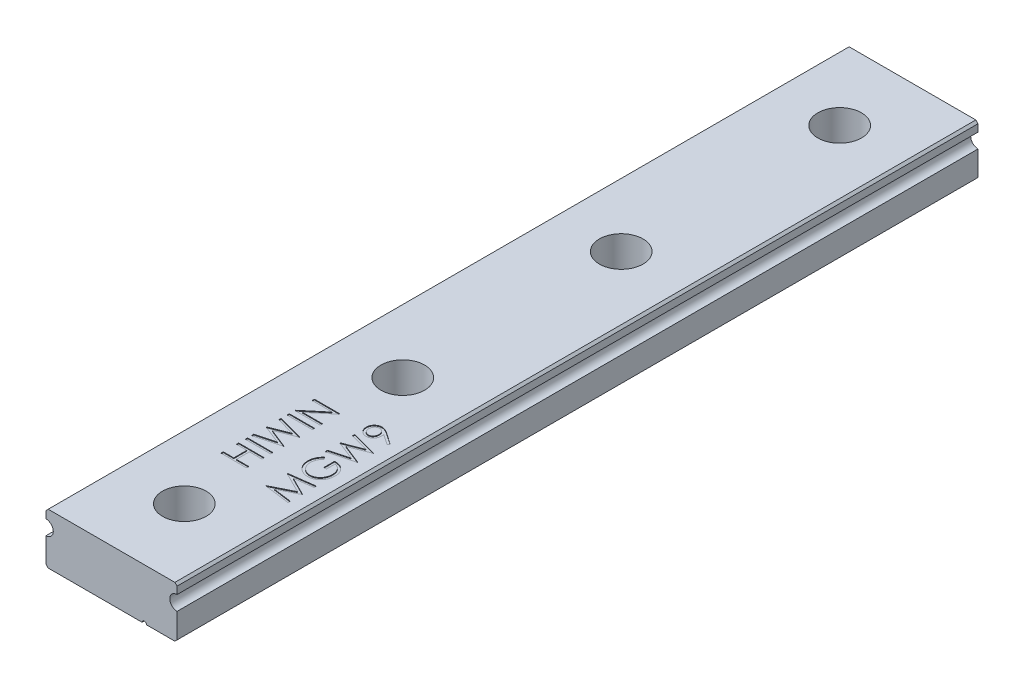
from build123d import *

# Parameters (mm, degrees)
BOSS_EXTRUDE1_DEPTH                                 = 110
CBORE_FOR_M3_HEX_SOCKET_HEAD_CAP_SCREW1_D           = 3.5
CBORE_FOR_M3_HEX_SOCKET_HEAD_CAP_SCREW1_CBORE_D     = 6
CBORE_FOR_M3_HEX_SOCKET_HEAD_CAP_SCREW1_CBORE_DEPTH = 4.5
LPATTERN1_COUNT                                     = 4
LPATTERN1_PITCH                                     = 30
SKETCH4_W                                           = 3.5
SKETCH4_H                                           = 0.314102564
CUT_EXTRUDE1_DEPTH                                  = 0.1


with BuildPart() as part:
    # Sketch1 → Boss-Extrude1 (new body)
    with BuildSketch(Plane.XY):
        with BuildLine():
            Line((9, 5.7), (9, 6.7))
            Line((9, 6.7), (8.7, 7))
            Line((8.7, 7), (-8.7, 7))
            Line((-8.7, 7), (-9, 6.7))
            Line((-9, 6.7), (-9, 5.7))
            ThreePointArc((-9, 5.7), (-8, 4.7), (-9, 3.7))
            Line((-9, 3.7), (-9, 0.3))
            Line((-9, 0.3), (-8.7, 0))
            Line((-8.7, 0), (4.2, 0))
            ThreePointArc((4.2, 0), (4.5, 0.3), (4.8, 0))
            Line((4.8, 0), (8.7, 0))
            Line((8.7, 0), (9, 0.3))
            Line((9, 0.3), (9, 3.7))
            ThreePointArc((9, 3.7), (8, 4.7), (9, 5.7))
        make_face()
    extrude(amount=-BOSS_EXTRUDE1_DEPTH)

    # CBORE for M3 Hex Socket Head Cap Screw1 (through all)
    with Locations(Plane(origin=(-0.084506888, 7, -67.993710711), x_dir=(-1, 0, 0), z_dir=(0, 1, 0))):
        with Locations((-0.084506888, 57.993710711)):
            cbore_for_m3_hex_socket_head_cap_screw1 = CounterBoreHole(CBORE_FOR_M3_HEX_SOCKET_HEAD_CAP_SCREW1_D / 2, CBORE_FOR_M3_HEX_SOCKET_HEAD_CAP_SCREW1_CBORE_D / 2, CBORE_FOR_M3_HEX_SOCKET_HEAD_CAP_SCREW1_CBORE_DEPTH)

    # LPattern1: CBORE for M3 Hex Socket Head Cap Screw1 ×4
    with Locations(*[(0, 0, -i * LPATTERN1_PITCH) for i in range(1, LPATTERN1_COUNT)]):
        add(cbore_for_m3_hex_socket_head_cap_screw1, mode=Mode.SUBTRACT)

    # Sketch4 → Cut-Extrude1 (cut)
    # profile 1 of 9: a face of its own
    with BuildSketch(Plane(origin=(0, 7, 0), x_dir=(1, 0, 0), z_dir=(0, 1, 0))):
        Polygon((-3.5, 18.538461538), (-3.5, 18.852564103), (-2.064102564, 18.852564103), (-2.064102564, 20.647435897), (-3.5, 20.647435897), (-3.5, 20.961538462), (0, 20.961538462), (0, 20.647435897), (-1.705128205, 20.647435897), (-1.705128205, 18.852564103), (0, 18.852564103), (0, 18.538461538), align=None)
    # profile 2 of 9: a face of its own
    with BuildSketch(Plane(origin=(0, 7, 0), x_dir=(1, 0, 0), z_dir=(0, 1, 0))):
        with Locations((-1.75, 22.016025641)):
            Rectangle(SKETCH4_W, SKETCH4_H)
    # profile 3 of 9: a face of its own
    with BuildSketch(Plane(origin=(0, 7, 0), x_dir=(1, 0, 0), z_dir=(0, 1, 0))):
        Polygon((-3.5, 22.711538462), (-3.5, 23.036157853), (-0.933193109, 23.721153846), (-3.5, 24.739883814), (-3.5, 24.785456731), (-0.950721154, 25.78525641), (-3.5, 26.473758013), (-3.5, 26.794871795), (0, 25.851161859), (0, 25.806290064), (-2.676883013, 24.753205128), (0, 23.6875), (0, 23.642628205), align=None)
    # profile 4 of 9: a face of its own
    with BuildSketch(Plane(origin=(0, 7, 0), x_dir=(1, 0, 0), z_dir=(0, 1, 0))):
        with Locations((-1.75, 27.759615385)):
            Rectangle(SKETCH4_W, SKETCH4_H)
    # profile 5 of 9: a face of its own
    with BuildSketch(Plane(origin=(0, 7, 0), x_dir=(1, 0, 0), z_dir=(0, 1, 0))):
        Polygon((0, 28.679487179), (-3.5, 28.679487179), (-3.5, 28.745392628), (-0.745292468, 31.057692308), (-3.5, 31.057692308), (-3.5, 31.371794872), (0, 31.371794872), (0, 31.300280449), (-2.748397436, 28.993589744), (0, 28.993589744), align=None)
    # profile 6 of 9: a face of its own
    with BuildSketch(Plane(origin=(0, 7, 0), x_dir=(1, 0, 0), z_dir=(0, 1, 0))):
        Polygon((6.967948718, 17.259615385), (3.467948718, 17.721654647), (3.467948718, 17.766526442), (6.33974359, 19.211538462), (3.467948718, 20.653044872), (3.467948718, 20.698617788), (6.967948718, 21.163461538), (6.967948718, 20.847956731), (4.449519231, 20.512820513), (6.967948718, 19.249399038), (6.967948718, 19.178585737), (4.443910256, 17.91025641), (6.967948718, 17.575821314), align=None)
    # profile 7 of 9: a face of its own
    with BuildSketch(Plane(origin=(0, 7, 0), x_dir=(1, 0, 0), z_dir=(0, 1, 0))):
        with BuildLine():
            Line((4.065304487, 25.157051282), (4.320512821, 24.887820513))
            add(Edge.make_bspline(
                [(4.320512821, 24.887820513), (4.274666598, 24.839111432), (4.184067383, 24.742854768), (4.066704644, 24.585654825), (3.965171715, 24.422298972), (3.883176125, 24.252523072), (3.818854464, 24.080779072), (3.7720985, 23.910020119), (3.742488341, 23.74135182), (3.738931922, 23.629187518), (3.737179487, 23.573918269)],
                knots=[0, 0, 0, 0, 1.089067066, 2.152164705, 3.18986567, 4.218445106, 5.218487318, 6.173592265, 7.100032889, 8, 8, 8, 8], degree=3))
            add(Edge.make_bspline(
                [(3.737179487, 23.573918269), (3.737593093, 23.540003569), (3.738419232, 23.472262129), (3.748963447, 23.371640185), (3.764128311, 23.272073548), (3.786070189, 23.173750173), (3.813879248, 23.076478886), (3.848664714, 22.980597998), (3.889219947, 22.885928627), (3.936082466, 22.793362608), (3.987562143, 22.703621874), (4.044611304, 22.618865878), (4.105397829, 22.538549416), (4.171457105, 22.464200209), (4.242141407, 22.395323695), (4.316177774, 22.330652995), (4.395021846, 22.271393416), (4.478349397, 22.218607776), (4.56422185, 22.170940182), (4.651910923, 22.129747982), (4.740602575, 22.093938028), (4.83096464, 22.066664067), (4.922065521, 22.043563193), (5.014382632, 22.027481957), (5.108157049, 22.01838564), (5.170954747, 22.016815149), (5.202524038, 22.016025641)],
                knots=[0, 0, 0, 0, 1.028150113, 2.053633673, 3.06513288, 4.081487945, 5.106702018, 6.131327874, 7.172780699, 8.228344599, 9.276313556, 10.308389736, 11.324843658, 12.329040066, 13.321460474, 14.316307835, 15.308626991, 16.309440696, 17.305625405, 18.28535951, 19.246194545, 20.203493668, 21.145557131, 22.095268976, 23.042464743, 24, 24, 24, 24], degree=3))
            add(Edge.make_bspline(
                [(5.202524038, 22.016025641), (5.2347947, 22.016781836), (5.299247902, 22.018292162), (5.395444304, 22.027945359), (5.490200886, 22.045900569), (5.583666689, 22.069712319), (5.676027725, 22.099984994), (5.767187608, 22.137177508), (5.857137476, 22.181483641), (5.944984394, 22.232654909), (6.030484526, 22.289164377), (6.111697005, 22.351315561), (6.187676723, 22.419213098), (6.259533466, 22.491612041), (6.326813744, 22.569172037), (6.388706596, 22.652645569), (6.446169075, 22.740864161), (6.498569911, 22.83386695), (6.545377278, 22.93067093), (6.587001488, 23.029927361), (6.621280742, 23.131955263), (6.649218868, 23.23621793), (6.672119159, 23.342591208), (6.686851641, 23.451615009), (6.697542472, 23.562487717), (6.698324142, 23.637226349), (6.698717949, 23.674879808)],
                knots=[0, 0, 0, 0, 0.935915162, 1.869274651, 2.799799983, 3.730201895, 4.664668062, 5.616159355, 6.583070886, 7.570012957, 8.562524459, 9.553461134, 10.53281078, 11.515274572, 12.509912756, 13.507571325, 14.526460018, 15.561318395, 16.601025881, 17.643204557, 18.680545676, 19.719612342, 20.772381578, 21.833430283, 22.908478249, 24, 24, 24, 24], degree=3))
            add(Edge.make_bspline(
                [(6.698717949, 23.674879808), (6.697769766, 23.72025834), (6.695907855, 23.80936646), (6.681401983, 23.94035028), (6.658775513, 24.066162898), (6.625536462, 24.186394736), (6.583464013, 24.301482131), (6.531435433, 24.411000619), (6.469998149, 24.515252613), (6.400396255, 24.613786873), (6.322847788, 24.704260894), (6.239913081, 24.786602973), (6.15051765, 24.857981595), (6.0559938, 24.920528912), (5.955437392, 24.972226156), (5.84940783, 25.014672034), (5.737839505, 25.047204491), (5.660747985, 25.060559579), (5.621794872, 25.067307692)],
                knots=[0, 0, 0, 0, 1.130199668, 2.219330667, 3.279027493, 4.311506524, 5.322739849, 6.327972234, 7.327472899, 8.33386792, 9.329086447, 10.29244429, 11.240784345, 12.174119183, 13.111530729, 14.052100829, 15.015757696, 16, 16, 16, 16], degree=3))
            Line((5.621794872, 25.067307692), (5.621794872, 23.900641026))
            Line((5.621794872, 23.900641026), (5.262820513, 23.900641026))
            Line((5.262820513, 23.900641026), (5.262820513, 25.381410256))
            add(Edge.make_bspline(
                [(5.262820513, 25.381410256), (5.329728002, 25.379704408), (5.460678043, 25.376365755), (5.651648314, 25.352946839), (5.832020008, 25.315130327), (6.001983079, 25.263470015), (6.161296672, 25.196594735), (6.310122538, 25.115222206), (6.447499219, 25.018050085), (6.574548223, 24.908539644), (6.687877435, 24.785639686), (6.787483373, 24.652671066), (6.871385988, 24.509414097), (6.93964665, 24.35600429), (6.992920645, 24.192943856), (7.030692222, 24.019855477), (7.053322185, 23.836973876), (7.056213565, 23.711637199), (7.057692308, 23.647536058)],
                knots=[0, 0, 0, 0, 1.140356446, 2.231883559, 3.274166699, 4.278491846, 5.25512956, 6.21435461, 7.1637429, 8.11826594, 9.068280886, 10.0076534, 10.945064095, 11.891975133, 12.864533718, 13.863980011, 14.907571808, 16, 16, 16, 16], degree=3))
            add(Edge.make_bspline(
                [(7.057692308, 23.647536058), (7.057123186, 23.608025922), (7.056000696, 23.530099201), (7.048023349, 23.415008273), (7.035742772, 23.303090653), (7.017197649, 23.194362644), (6.994482995, 23.088424302), (6.965396276, 22.985804717), (6.931727576, 22.886112975), (6.893431903, 22.789194989), (6.849060246, 22.695930442), (6.799750607, 22.605903925), (6.745757246, 22.5186178), (6.6861464, 22.434666635), (6.62136394, 22.353613013), (6.551280021, 22.27597957), (6.476108901, 22.201331692), (6.422729892, 22.154571228), (6.395833333, 22.131009615)],
                knots=[0, 0, 0, 0, 1.107784379, 2.184907829, 3.233506516, 4.263428166, 5.276301166, 6.270063455, 7.25232949, 8.225834625, 9.190232166, 10.146266622, 11.1027726, 12.066435141, 13.031522626, 14.010570082, 14.99756817, 16, 16, 16, 16], degree=3))
            add(Edge.make_bspline(
                [(6.395833333, 22.131009615), (6.35316268, 22.096823683), (6.268529663, 22.029019271), (6.132929719, 21.941741114), (5.992527859, 21.867339711), (5.84693323, 21.806971889), (5.696282017, 21.759833803), (5.540766726, 21.72602755), (5.380187096, 21.706220261), (5.271521831, 21.703366724), (5.216546474, 21.701923077)],
                knots=[0, 0, 0, 0, 1.023165419, 2.029347347, 3.013907458, 3.994755782, 4.975994455, 5.96558838, 6.970761222, 8, 8, 8, 8], degree=3))
            add(Edge.make_bspline(
                [(5.216546474, 21.701923077), (5.175380222, 21.702455315), (5.093570914, 21.703513027), (4.972113608, 21.716338544), (4.85281291, 21.734739957), (4.735766374, 21.761787032), (4.620895706, 21.795883218), (4.508148028, 21.838436999), (4.397455075, 21.887980777), (4.289585288, 21.945570494), (4.185945674, 22.009639231), (4.087043404, 22.079246887), (3.994481386, 22.154930572), (3.908045197, 22.236910667), (3.826453743, 22.323534597), (3.751411343, 22.416620898), (3.681743707, 22.514759234), (3.618789497, 22.618710374), (3.562221643, 22.726834005), (3.512633564, 22.838895091), (3.471649942, 22.954852909), (3.436876246, 23.073840466), (3.411161083, 23.196757945), (3.392512344, 23.322713488), (3.379751742, 23.452363598), (3.378725487, 23.539999628), (3.378205128, 23.584435096)],
                knots=[0, 0, 0, 0, 1.00895651, 2.005089799, 2.991467152, 3.967318338, 4.948153826, 5.927364234, 6.919980553, 7.91976625, 8.923240147, 9.905815003, 10.88314567, 11.851989312, 12.825009789, 13.798721852, 14.781296708, 15.773896486, 16.776076962, 17.771600213, 18.775744723, 19.78957137, 20.808953803, 21.851964491, 22.910847925, 24, 24, 24, 24], degree=3))
            add(Edge.make_bspline(
                [(3.378205128, 23.584435096), (3.37878462, 23.62067334), (3.379933684, 23.692529519), (3.387898332, 23.799455251), (3.400522213, 23.904728266), (3.417749, 24.008504655), (3.44121269, 24.110431022), (3.469290975, 24.210797727), (3.501982797, 24.309750263), (3.540971644, 24.406978512), (3.585225269, 24.503136228), (3.635038691, 24.598758069), (3.691263696, 24.693517315), (3.754067231, 24.787578296), (3.822370649, 24.881534154), (3.898127473, 24.973898797), (3.978350229, 25.066901741), (4.036032413, 25.126703555), (4.065304487, 25.157051282)],
                knots=[0, 0, 0, 0, 0.985871117, 1.954866573, 2.915460327, 3.869826059, 4.81536089, 5.759505086, 6.70452669, 7.649098992, 8.607881297, 9.583363685, 10.581137262, 11.603961102, 12.659522466, 13.73993555, 14.853081303, 16, 16, 16, 16], degree=3))
        make_face()
    # profile 8 of 9: a face of its own
    with BuildSketch(Plane(origin=(0, 7, 0), x_dir=(1, 0, 0), z_dir=(0, 1, 0))):
        Polygon((3.467948718, 25.875), (3.467948718, 26.199619391), (6.034755609, 26.884615385), (3.467948718, 27.903345353), (3.467948718, 27.948918269), (6.017227564, 28.948717949), (3.467948718, 29.637219551), (3.467948718, 29.958333333), (6.967948718, 29.014623397), (6.967948718, 28.969751603), (4.291065705, 27.916666667), (6.967948718, 26.850961538), (6.967948718, 26.806089744), align=None)
    # profile 9 of 9: a face of its own
    with BuildSketch(Plane(origin=(0, 7, 0), x_dir=(1, 0, 0), z_dir=(0, 1, 0))):
        with BuildLine():
            Line((7.057692308, 31.21474359), (6.883112981, 30.963741987))
            Line((6.883112981, 30.963741987), (5.460536859, 31.936899038))
            add(Edge.make_bspline(
                [(5.460536859, 31.936899038), (5.468484228, 31.874816887), (5.484128885, 31.752606126), (5.486173514, 31.629419057), (5.487179487, 31.568810096)],
                knots=[0, 0, 0, 0, 1.015985029, 2, 2, 2, 2], degree=3))
            add(Edge.make_bspline(
                [(5.487179487, 31.568810096), (5.486238411, 31.532068048), (5.48439116, 31.459946622), (5.469749352, 31.353914968), (5.447199222, 31.252029412), (5.413550474, 31.154560041), (5.371732239, 31.061140592), (5.319875323, 30.971974669), (5.258868658, 30.887183581), (5.189037089, 30.807673113), (5.112353766, 30.735372706), (5.031217129, 30.670908546), (4.944751315, 30.617625601), (4.854779905, 30.572573239), (4.759382554, 30.539364355), (4.660177979, 30.514597119), (4.556550375, 30.499515979), (4.486027439, 30.497711216), (4.450220353, 30.496794872)],
                knots=[0, 0, 0, 0, 1.060698949, 2.082059282, 3.085738422, 4.069684654, 5.054463875, 6.037298355, 7.043153692, 8.066652628, 9.088369706, 10.083456696, 11.053578809, 12.016466116, 12.983507685, 13.964045196, 14.966270913, 16, 16, 16, 16], degree=3))
            add(Edge.make_bspline(
                [(4.450220353, 30.496794872), (4.401253588, 30.498532793), (4.305141762, 30.501943978), (4.164681125, 30.529292887), (4.031796079, 30.57460498), (3.906635217, 30.636793474), (3.792073486, 30.716623684), (3.688499026, 30.811427974), (3.597759456, 30.921972578), (3.519848855, 31.04537136), (3.456761609, 31.178548236), (3.411940809, 31.31860434), (3.383308236, 31.463180339), (3.3799135, 31.561432729), (3.378205128, 31.610877404)],
                knots=[0, 0, 0, 0, 1.023011052, 2.007963168, 2.978169221, 3.950402619, 4.919353283, 5.887490769, 6.876420893, 7.899700203, 8.931203047, 9.947778163, 10.96723692, 12, 12, 12, 12], degree=3))
            add(Edge.make_bspline(
                [(3.378205128, 31.610877404), (3.380035301, 31.659365807), (3.383651551, 31.755174323), (3.410135375, 31.896063561), (3.454772592, 32.031003704), (3.516455108, 32.159251982), (3.593783616, 32.277979178), (3.685890325, 32.3847997), (3.792852151, 32.476878922), (3.911730876, 32.555383638), (4.040246296, 32.617227218), (4.174138011, 32.66254286), (4.312600654, 32.690242692), (4.406391902, 32.693745196), (4.453725962, 32.695512821)],
                knots=[0, 0, 0, 0, 1.026358223, 2.027987109, 3.023239252, 4.028077889, 5.032770297, 6.015020143, 7.004250571, 8.011656937, 9.02310243, 10.015224881, 10.998334443, 12, 12, 12, 12], degree=3))
            add(Edge.make_bspline(
                [(4.453725962, 32.695512821), (4.490468378, 32.694329163), (4.564991178, 32.69192841), (4.678017661, 32.675308171), (4.793168632, 32.646639359), (4.890727756, 32.614605929), (4.971550238, 32.583207772), (5.035581535, 32.554505227), (5.102509069, 32.521163256), (5.172606902, 32.483926368), (5.245966492, 32.442865108), (5.322079032, 32.396863244), (5.401055492, 32.346541246), (5.454303784, 32.310713843), (5.481570513, 32.292367788)],
                knots=[0, 0, 0, 0, 1.179894106, 2.393120058, 3.660107319, 4.986885617, 5.687958251, 6.443931318, 7.239444731, 8.088894906, 8.992865148, 9.938946712, 10.944601238, 12, 12, 12, 12], degree=3))
            Line((5.481570513, 32.292367788), (7.057692308, 31.21474359))
        make_face()
        with BuildLine():
            add(Edge.make_bspline(
                [(5.128205128, 31.627003205), (5.127443169, 31.654836551), (5.125959894, 31.709018613), (5.116972501, 31.788405182), (5.10091985, 31.86329601), (5.078251267, 31.934173102), (5.049534697, 32.000950651), (5.014538857, 32.063649693), (4.97249706, 32.121629784), (4.925241239, 32.175097344), (4.873450736, 32.223620781), (4.817962021, 32.265459166), (4.760498938, 32.301683637), (4.699885133, 32.330582666), (4.637112179, 32.353872325), (4.571272257, 32.370123036), (4.502819953, 32.379098526), (4.456321832, 32.380631318), (4.432692308, 32.381410256)],
                knots=[0, 0, 0, 0, 1.163726718, 2.265380301, 3.334713825, 4.36057981, 5.371541381, 6.368955992, 7.355979581, 8.359691305, 9.348261197, 10.317521986, 11.261029684, 12.183096459, 13.119698615, 14.055740009, 15.011961376, 16, 16, 16, 16], degree=3))
            add(Edge.make_bspline(
                [(4.432692308, 32.381410256), (4.409052319, 32.380741236), (4.362466821, 32.37942285), (4.293921732, 32.368826223), (4.228211162, 32.350235718), (4.164887772, 32.325039313), (4.104297734, 32.292476775), (4.04625008, 32.253022786), (3.991623454, 32.205381257), (3.939517566, 32.152143972), (3.892248709, 32.093589326), (3.850485484, 32.031550316), (3.815239605, 31.966358363), (3.787407408, 31.897722647), (3.764606292, 31.82657522), (3.748465177, 31.752179536), (3.739472619, 31.674432778), (3.7379536, 31.621650296), (3.737179487, 31.594751603)],
                knots=[0, 0, 0, 0, 0.971910406, 1.91526867, 2.84337505, 3.775008003, 4.712374136, 5.666733183, 6.654995996, 7.688089235, 8.726800303, 9.745078658, 10.75990398, 11.768337501, 12.786615857, 13.829099629, 14.893678693, 16, 16, 16, 16], degree=3))
            add(Edge.make_bspline(
                [(3.737179487, 31.594751603), (3.737954872, 31.568086848), (3.739476172, 31.515770819), (3.748447901, 31.438715191), (3.764715942, 31.364822663), (3.787397076, 31.293881759), (3.815241735, 31.225248032), (3.850487343, 31.160059153), (3.892239015, 31.09800569), (3.939555202, 31.039506747), (3.99138048, 30.986173509), (4.046494174, 30.939338145), (4.104267004, 30.899794933), (4.164895888, 30.867277883), (4.228209004, 30.842069447), (4.293922316, 30.823482154), (4.362466669, 30.812884664), (4.409052268, 30.811566396), (4.432692308, 30.810897436)],
                knots=[0, 0, 0, 0, 1.099107991, 2.156440826, 3.191784126, 4.212280276, 5.222910149, 6.239945746, 7.260441896, 8.30141526, 9.33675856, 10.320924759, 11.277362386, 12.216770088, 13.150432123, 14.080559904, 15.025972789, 16, 16, 16, 16], degree=3))
            add(Edge.make_bspline(
                [(4.432692308, 30.810897436), (4.456340163, 30.81150402), (4.502978061, 30.812700315), (4.571509405, 30.824218625), (4.637179138, 30.843532257), (4.700547843, 30.869142235), (4.760795693, 30.903511564), (4.818235099, 30.945280238), (4.874040333, 30.993474159), (4.925079304, 31.049672747), (4.972723236, 31.110020312), (5.014274516, 31.174840024), (5.04911654, 31.242829298), (5.078335917, 31.313551594), (5.100691189, 31.387536106), (5.116942683, 31.464679812), (5.125873731, 31.544996604), (5.12742054, 31.599405412), (5.128205128, 31.627003205)],
                knots=[0, 0, 0, 0, 0.952872936, 1.879239831, 2.791748947, 3.708674669, 4.628500839, 5.580394867, 6.568761142, 7.595635223, 8.636123962, 9.665976811, 10.694276597, 11.712685318, 12.747011694, 13.805940053, 14.887106426, 16, 16, 16, 16], degree=3))
        make_face(mode=Mode.SUBTRACT)
    extrude(amount=-CUT_EXTRUDE1_DEPTH, mode=Mode.SUBTRACT)


solid = part.part
